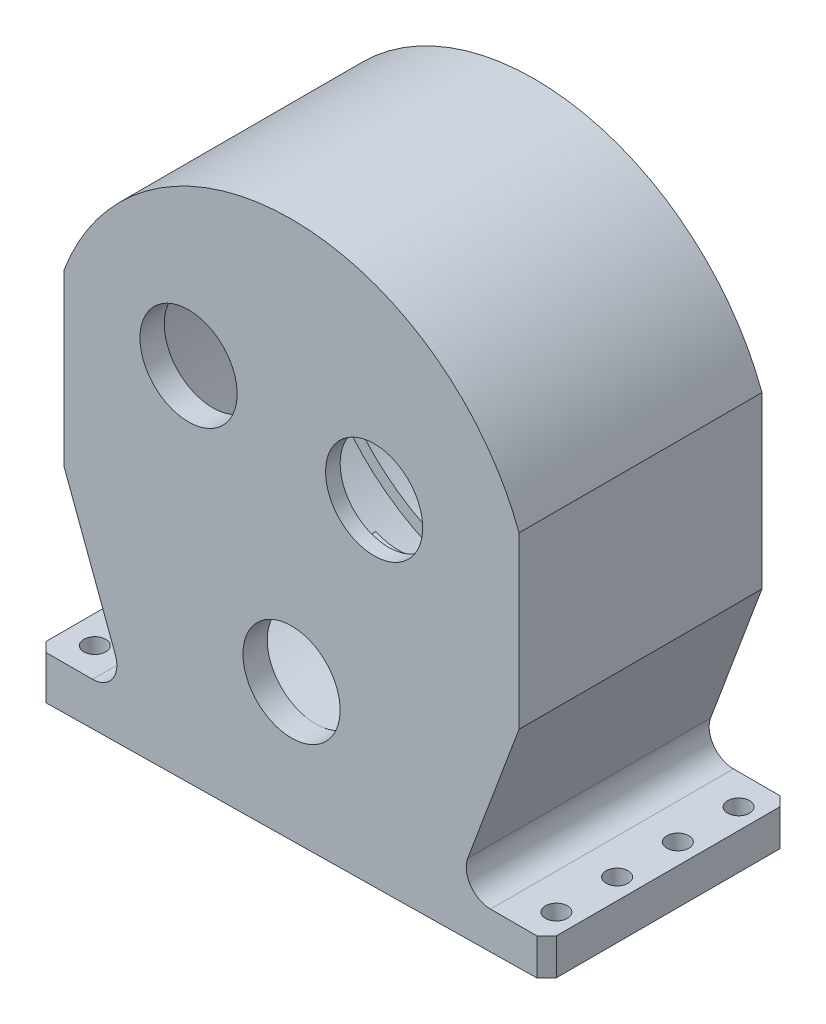
from build123d import *

# Parameters (mm, degrees)
SKETCH1_R           = 50
BOSS_EXTRUDE1_DEPTH = 50
SKETCH2_R           = 42.5
CUT_EXTRUDE1_DEPTH  = 45
SKETCH3_R           = 12.5
CUT_EXTRUDE2_DEPTH  = 2
SKETCH4_R           = 10
CUT_EXTRUDE3_DEPTH  = 84.815273071
BOSS_EXTRUDE2_DEPTH = 50
CUT_EXTRUDE4_DEPTH  = 96.077733998
SKETCH7_R           = 2.25
CUT_EXTRUDE5_DEPTH  = 20
FILLET1_R           = 5
FILLET2_R           = 5
CHAMFER1_SIZE       = 2
SKETCH8_R           = 4
CUT_EXTRUDE6_DEPTH  = 1
SKETCH9_R           = 11.5
CUT_EXTRUDE8_DEPTH  = 2
SKETCH10_R          = 42.5
SKETCH10_R_2        = 40
BOSS_EXTRUDE3_DEPTH = 5
SKETCH11_R          = 2
CUT_EXTRUDE9_DEPTH  = 8


with BuildPart() as part:
    # Sketch1 → Boss-Extrude1 (new body)
    with BuildSketch(Plane.XY):
        Circle(SKETCH1_R)
    extrude(amount=BOSS_EXTRUDE1_DEPTH)

    # Sketch2 → Cut-Extrude1 (cut)
    with BuildSketch(Plane(origin=(0, 0, 0), x_dir=(-1, 0, 0), z_dir=(0, 0, -1))):
        Circle(SKETCH2_R)
    extrude(amount=-CUT_EXTRUDE1_DEPTH, mode=Mode.SUBTRACT)

    # Sketch3 → Cut-Extrude2 (cut)
    with BuildSketch(Plane(origin=(0, 0, 45), x_dir=(-1, 0, 0), z_dir=(0, 0, -1))):
        Circle(SKETCH3_R)
    extrude(amount=-CUT_EXTRUDE2_DEPTH, mode=Mode.SUBTRACT)

    # Sketch4 → Cut-Extrude3 (cut, through all)
    with BuildSketch(Plane(origin=(0, 0, 45), x_dir=(-1, 0, 0), z_dir=(0, 0, -1))):
        with Locations((-17, 8.485281374)):
            Circle(SKETCH4_R)
        with Locations((21.2, 13.24990566)):
            Circle(SKETCH4_R)
        with Locations((0, -32.5)):
            Circle(SKETCH4_R)
    extrude(amount=-CUT_EXTRUDE3_DEPTH, mode=Mode.SUBTRACT)

    # Sketch5 → Boss-Extrude2 (add)
    with BuildSketch(Plane(origin=(0, 0, 0), x_dir=(-1, 0, 0), z_dir=(0, 0, -1))):
        with BuildLine():
            Line((-46.833609462, -17.510369063), (-33.74764568, -52.510369063))
            Line((-33.74764568, -52.510369063), (-52.5, -52.510369063))
            Line((-52.5, -52.510369063), (-52.5, -59.989582371))
            Line((-52.5, -59.989582371), (52.5, -61.510369063))
            Line((52.5, -61.510369063), (52.5, -52.510369063))
            Line((52.5, -52.510369063), (33.74764568, -52.510369063))
            Line((33.74764568, -52.510369063), (46.833609462, -17.510369063))
            ThreePointArc((46.833609462, -17.510369063), (0, -50), (-46.833609462, -17.510369063))
        make_face()
    extrude(amount=-BOSS_EXTRUDE2_DEPTH)

    # Sketch6 → Cut-Extrude4 (cut, through all)
    with BuildSketch(Plane(origin=(0, 0, 0), x_dir=(-1, 0, 0), z_dir=(0, 0, -1))):
        with BuildLine():
            Line((-46.833609462, -17.510369063), (-46.833609462, 17.510369063))
            ThreePointArc((-46.833609462, 17.510369063), (-50, 0), (-46.833609462, -17.510369063))
        make_face()
        with BuildLine():
            Line((46.833609462, -17.510369063), (46.833609462, 17.510369063))
            ThreePointArc((46.833609462, 17.510369063), (50, 0), (46.833609462, -17.510369063))
        make_face()
    extrude(amount=-CUT_EXTRUDE4_DEPTH, mode=Mode.SUBTRACT)

    # Sketch7 → Cut-Extrude5 (cut)
    with BuildSketch(Plane(origin=(0.879698836, -60.737234438, 0), x_dir=(0.9998951279661363, 0.014482163843290402, 0), z_dir=(0.014482163843290404, -0.9998951279661364, 0))):
        with Locations((-47.5, 43.75)):
            Circle(SKETCH7_R)
        with Locations((-47.5, 31.25)):
            Circle(SKETCH7_R)
        with Locations((47.5, 31.25)):
            Circle(SKETCH7_R)
        with Locations((47.5, 43.75)):
            Circle(SKETCH7_R)
        with Locations((47.5, 18.75)):
            Circle(SKETCH7_R)
        with Locations((47.5, 6.25)):
            Circle(SKETCH7_R)
        with Locations((-47.5, 18.75)):
            Circle(SKETCH7_R)
        with Locations((-47.5, 6.25)):
            Circle(SKETCH7_R)
    extrude(amount=-CUT_EXTRUDE5_DEPTH, mode=Mode.SUBTRACT)

    # Fillet1
    fillet1_edges = [part.edges().sort_by_distance(p)[0] for p in [
        (33.74764568, -52.510369063, 25),
    ]]
    fillet(fillet1_edges, radius=FILLET1_R)

    # Fillet2
    fillet2_edges = [part.edges().sort_by_distance(p)[0] for p in [
        (-33.74764568, -52.510369063, 25),
    ]]
    fillet(fillet2_edges, radius=FILLET2_R)

    # Chamfer1
    chamfer1_edges = [part.edges().sort_by_distance(p)[0] for p in [
        (-52.5, -57.010369063, 50),
        (52.5, -56.249975717, 50),
        (52.5, -56.249975717, 0),
        (-52.5, -57.010369063, 0),
    ]]
    chamfer(chamfer1_edges, length=CHAMFER1_SIZE)

    # Sketch8 → Cut-Extrude6 (cut)
    with BuildSketch(Plane(origin=(0, 0, 47), x_dir=(-1, 0, 0), z_dir=(0, 0, -1))):
        Circle(SKETCH8_R)
    extrude(amount=-CUT_EXTRUDE6_DEPTH, mode=Mode.SUBTRACT)

    # Sketch9 → Cut-Extrude8 (cut)
    with BuildSketch(Plane(origin=(0, 0, 45), x_dir=(-1, 0, 0), z_dir=(0, 0, -1))):
        with Locations((-17, 8.485281374)):
            Circle(SKETCH9_R)
    extrude(amount=-CUT_EXTRUDE8_DEPTH, mode=Mode.SUBTRACT)

    # Sketch10 → Boss-Extrude3 (add)
    with BuildSketch(Plane(origin=(0, 0, 0), x_dir=(-1, 0, 0), z_dir=(0, 0, -1))):
        Circle(SKETCH10_R)
        Circle(SKETCH10_R_2, mode=Mode.SUBTRACT)
    extrude(amount=-BOSS_EXTRUDE3_DEPTH)

    # Sketch11 → Cut-Extrude9 (cut)
    with BuildSketch(Plane(origin=(0, 0, 0), x_dir=(-1, 0, 0), z_dir=(0, 0, -1))):
        with Locations((0, 46)):
            Circle(SKETCH11_R)
        with Locations((23, 39.837168574)):
            Circle(SKETCH11_R)
        with Locations((39.837168574, 23)):
            Circle(SKETCH11_R)
        with Locations((-23, 39.837168574)):
            Circle(SKETCH11_R)
        with Locations((-39.837168574, 23)):
            Circle(SKETCH11_R)
        with Locations(Location((39.837168574, -23, 0), (0, 0, 180))):
            Circle(SKETCH11_R)
        with Locations(Location((23, -39.837168574, 0), (0, 0, 180))):
            Circle(SKETCH11_R)
        with Locations(Location((0, -46, 0), (0, 0, 180))):
            Circle(SKETCH11_R)
        with Locations(Location((-23, -39.837168574, 0), (0, 0, 180))):
            Circle(SKETCH11_R)
        with Locations(Location((-39.837168574, -23, 0), (0, 0, 180))):
            Circle(SKETCH11_R)
    extrude(amount=-CUT_EXTRUDE9_DEPTH, mode=Mode.SUBTRACT)


solid = part.part
